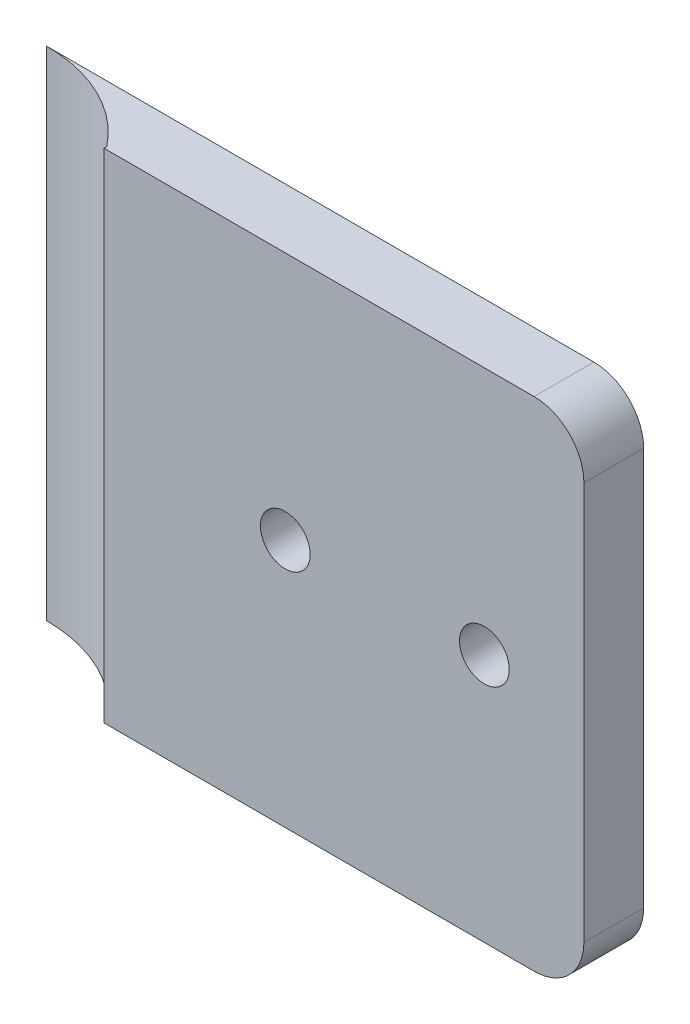
SolidWorks part; units mm, degrees
material "1023 碳钢板 (SS)"
ref_plane "Front Plane" through (0, 0, 0) normal (0, 0, 1) x (1, 0, 0)
ref_plane "Top Plane" through (0, 0, 0) normal (0, 1, 0) x (1, 0, 0)
ref_plane "Right Plane" through (0, 0, 0) normal (1, 0, 0) x (0, 0, -1)
ref_plane "Plane1" through (0, 0, -15) normal (0, 0, 1) x (1, 0, 0)
sketch "Sketch1" plane through (0, 0, -15) normal (0, 0, 1) x (1, 0, 0)
  line L0 (11.8, -210) -> (11.8, 210) construction
  line L1 (11.8, -5) -> (55, -5)
  line L2 (11.8, -5) -> (11.8, -55)
  line L3 (11.8, -55) -> (55, -55)
  line L4 (60, -10) -> (60, -50)
  line L5 (15, 210) -> (-15, 210) construction
  arc A0 (60, -50) -> (55, -55) centre (55, -50) cw
  arc A1 (55, -5) -> (60, -10) centre (55, -10) cw
  point P11 (60, -55)
  point P14 (60, -5)
  dimension "D4" = 5
  dimension "D1" = 60
  dimension "D2" = 50
  dimension "D3" = 215
extrude "Boss-Extrude1" add sketch "Sketch1" along normal blind 6
sketch "Sketch2" plane through (0, -5, 0) normal (0, 1, 0) x (1, 0, 0)
  line L0 (0, 15) -> (11.8, 15)
  line L1 (11.8, 15) -> (11.8, 9.2607)
  circle A0 centre (0, 0) radius 15 construction
  arc A1 (11.8, 9.2607) -> (0, 15) centre (0, 0) ccw
extrude "Boss-Extrude2" add sketch "Sketch2" against normal up to surface (50 mm away) up to face at (33.4, -55, -12)
hole_wizard "M6 Tapped Hole1" positions "3DSketch1" profile "Sketch3" tap size "M6" standard "IS"
sketch3d "3DSketch1"
  line L0 (60, -50, -9) -> (60, -10, -9) construction
  line L1 (55, -5, -9) -> (11.8, -5, -9) construction
  point P0 (50, -30, -9)
  point P2 (30, -30, -9)
  dimension "D1" = 10
  dimension "D2" = 20
  dimension "D3" = 25
  dimension "D4" = 25
sketch "Sketch3" plane through (50, -30, -9) normal (1, 0, 0) x (0, -1, 0)
  line L0 (0, 0) -> (0, 16.5022)
  line L1 (0, 16.5022) -> (2.5, 15)
  line L2 (2.5, 15) -> (2.5, 0)
  line L5 (2.5, 0) -> (0, 0)
  line L10 (0, 16.5022) -> (-2.5, 15) construction
  line L11 (0, -6.35) -> (0, 107.95) construction
  dimension "螺纹孔钻头直径" = 5
  dimension "螺纹孔钻头深度" = 15
  dimension "导头角度" = 118
cosmetic thread "Cosmetic thread 1" parameters "D1"=12, "D2"=6
cosmetic thread "Cosmetic thread 2" parameters "D1"=12, "D2"=6
